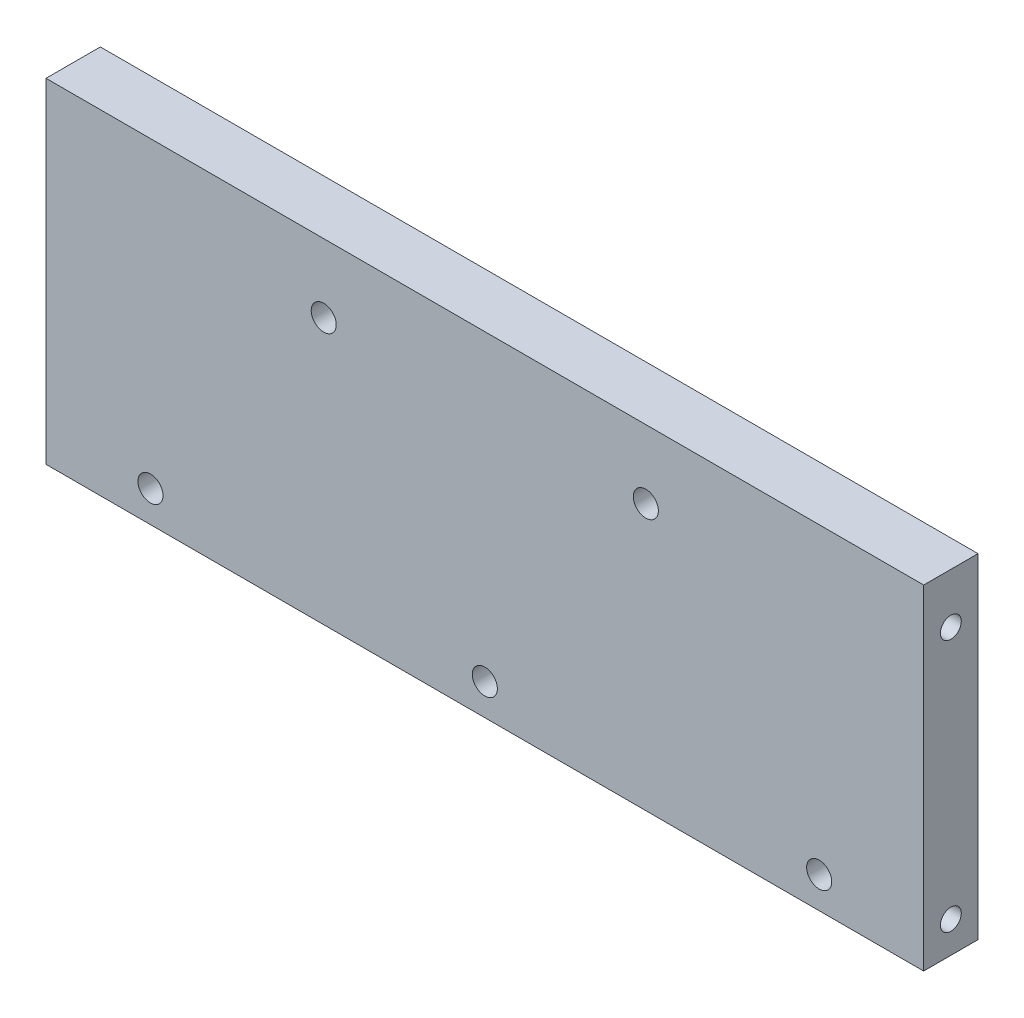
from build123d import *

# Parameters (mm, degrees)
SKETCH1_W                 = 210
SKETCH1_H                 = 80
BOSS_EXTRUDE1_DEPTH       = 13
SKETCH2_R                 = 5
SKETCH2_R_2               = 3
CUT_EXTRUDE1_DEPTH        = 6
CUT_EXTRUDE2_REACH        = 115.111
SKETCH2_5_R               = 3
M6X1_0_TAPPED_HOLE1_D     = 5
M6X1_0_TAPPED_HOLE1_DEPTH = 15
M6X1_0_TAPPED_HOLE1_TIP   = 1.502151548
SKETCH8_R                 = 5
SKETCH8_R_2               = 3
CUT_EXTRUDE3_DEPTH        = 6
CUT_EXTRUDE4_REACH        = 115.111
SKETCH8_4_R               = 3
M6X1_0_TAPPED_HOLE2_D     = 5
M6X1_0_TAPPED_HOLE2_DEPTH = 15
M6X1_0_TAPPED_HOLE2_TIP   = 1.502151548


with BuildPart() as part:
    # Sketch1 → Boss-Extrude1 (new body)
    with BuildSketch(Plane.XY):
        Rectangle(SKETCH1_W, SKETCH1_H)
    extrude(amount=BOSS_EXTRUDE1_DEPTH)

    # Sketch2 → Cut-Extrude1 (cut)
    # profile 1 of 2: a face of its own
    with BuildSketch(Plane(origin=(0, 0, 0), x_dir=(-1, 0, 0), z_dir=(0, 0, -1))):
        with Locations((-38.524202037, 23.616817232)):
            Circle(SKETCH2_R)
        with Locations((-38.524202037, 23.616817232)):
            Circle(SKETCH2_R_2, mode=Mode.SUBTRACT)
    # profile 2 of 2: a face of its own
    with BuildSketch(Plane(origin=(0, 0, 0), x_dir=(-1, 0, 0), z_dir=(0, 0, -1))):
        with Locations((38.548404074, 23.616912244)):
            Circle(SKETCH2_R)
        with Locations((38.548404074, 23.616912244)):
            Circle(SKETCH2_R_2, mode=Mode.SUBTRACT)
    extrude(amount=-CUT_EXTRUDE1_DEPTH, mode=Mode.SUBTRACT)

    # Sketch2<5> → Cut-Extrude2 (cut, up to next)
    with BuildSketch(Plane(origin=(0, 0, 0), x_dir=(-1, 0, 0), z_dir=(0, 0, -1)), mode=Mode.PRIVATE) as cut_extrude2_sk1:
        with Locations((-38.524202037, 23.616817232)):
            Circle(SKETCH2_5_R)
    cut_extrude2_tool1 = extrude(cut_extrude2_sk1.sketch, amount=-CUT_EXTRUDE2_REACH, mode=Mode.PRIVATE) & part.part
    # Sketch2<5> → Cut-Extrude2 (cut, up to next)
    with BuildSketch(Plane(origin=(0, 0, 0), x_dir=(-1, 0, 0), z_dir=(0, 0, -1)), mode=Mode.PRIVATE) as cut_extrude2_sk2:
        with Locations((38.548404074, 23.616912244)):
            Circle(SKETCH2_5_R)
    cut_extrude2_tool2 = extrude(cut_extrude2_sk2.sketch, amount=-CUT_EXTRUDE2_REACH, mode=Mode.PRIVATE) & part.part
    add(cut_extrude2_tool1.solids().sort_by_distance((38.524202, 23.616817, 0))[0], mode=Mode.SUBTRACT)
    add(cut_extrude2_tool2.solids().sort_by_distance((-38.548404, 23.616912, 0))[0], mode=Mode.SUBTRACT)

    # M6x1.0 Tapped Hole1
    with Locations(Plane(origin=(105, -32.5, 6.5), x_dir=(0, 0, 1), z_dir=(1, 0, 0))):
        with Locations((0, 0)):
            Hole(M6X1_0_TAPPED_HOLE1_D / 2, depth=M6X1_0_TAPPED_HOLE1_DEPTH)
            with Locations((0, 0, -(M6X1_0_TAPPED_HOLE1_DEPTH + M6X1_0_TAPPED_HOLE1_TIP / 2))):  # 118° drill point
                Cone(0, M6X1_0_TAPPED_HOLE1_D / 2, M6X1_0_TAPPED_HOLE1_TIP, mode=Mode.SUBTRACT)

    # Sketch8 → Cut-Extrude3 (cut)
    # profile 1 of 3: a face of its own
    with BuildSketch(Plane(origin=(0, 0, 0), x_dir=(-1, 0, 0), z_dir=(0, 0, -1))):
        with Locations((-80, -32.5)):
            Circle(SKETCH8_R)
        with Locations((-80, -32.5)):
            Circle(SKETCH8_R_2, mode=Mode.SUBTRACT)
    # profile 2 of 3: a face of its own
    with BuildSketch(Plane(origin=(0, 0, 0), x_dir=(-1, 0, 0), z_dir=(0, 0, -1))):
        with Locations((80, -32.5)):
            Circle(SKETCH8_R)
        with Locations((80, -32.5)):
            Circle(SKETCH8_R_2, mode=Mode.SUBTRACT)
    # profile 3 of 3: a face of its own
    with BuildSketch(Plane(origin=(0, 0, 0), x_dir=(-1, 0, 0), z_dir=(0, 0, -1))):
        with Locations((0, -32.5)):
            Circle(SKETCH8_R)
        with Locations((0, -32.5)):
            Circle(SKETCH8_R_2, mode=Mode.SUBTRACT)
    extrude(amount=-CUT_EXTRUDE3_DEPTH, mode=Mode.SUBTRACT)

    # Sketch8<4> → Cut-Extrude4 (cut, up to next)
    with BuildSketch(Plane(origin=(0, 0, 0), x_dir=(-1, 0, 0), z_dir=(0, 0, -1)), mode=Mode.PRIVATE) as cut_extrude4_sk1:
        with Locations((-80, -32.5)):
            Circle(SKETCH8_4_R)
    cut_extrude4_tool1 = extrude(cut_extrude4_sk1.sketch, amount=-CUT_EXTRUDE4_REACH, mode=Mode.PRIVATE) & part.part
    # Sketch8<4> → Cut-Extrude4 (cut, up to next)
    with BuildSketch(Plane(origin=(0, 0, 0), x_dir=(-1, 0, 0), z_dir=(0, 0, -1)), mode=Mode.PRIVATE) as cut_extrude4_sk2:
        with Locations((0, -32.5)):
            Circle(SKETCH8_4_R)
    cut_extrude4_tool2 = extrude(cut_extrude4_sk2.sketch, amount=-CUT_EXTRUDE4_REACH, mode=Mode.PRIVATE) & part.part
    # Sketch8<4> → Cut-Extrude4 (cut, up to next)
    with BuildSketch(Plane(origin=(0, 0, 0), x_dir=(-1, 0, 0), z_dir=(0, 0, -1)), mode=Mode.PRIVATE) as cut_extrude4_sk3:
        with Locations((80, -32.5)):
            Circle(SKETCH8_4_R)
    cut_extrude4_tool3 = extrude(cut_extrude4_sk3.sketch, amount=-CUT_EXTRUDE4_REACH, mode=Mode.PRIVATE) & part.part
    add(cut_extrude4_tool1.solids().sort_by_distance((80, -32.5, 0))[0], mode=Mode.SUBTRACT)
    add(cut_extrude4_tool2.solids().sort_by_distance((0, -32.5, 0))[0], mode=Mode.SUBTRACT)
    add(cut_extrude4_tool3.solids().sort_by_distance((-80, -32.5, 0))[0], mode=Mode.SUBTRACT)

    # M6x1.0 Tapped Hole2
    with Locations(Plane(origin=(105, 28, 6.5), x_dir=(0, 0, 1), z_dir=(1, 0, 0))):
        with Locations((0, 0)):
            Hole(M6X1_0_TAPPED_HOLE2_D / 2, depth=M6X1_0_TAPPED_HOLE2_DEPTH)
            with Locations((0, 0, -(M6X1_0_TAPPED_HOLE2_DEPTH + M6X1_0_TAPPED_HOLE2_TIP / 2))):  # 118° drill point
                Cone(0, M6X1_0_TAPPED_HOLE2_D / 2, M6X1_0_TAPPED_HOLE2_TIP, mode=Mode.SUBTRACT)


solid = part.part
